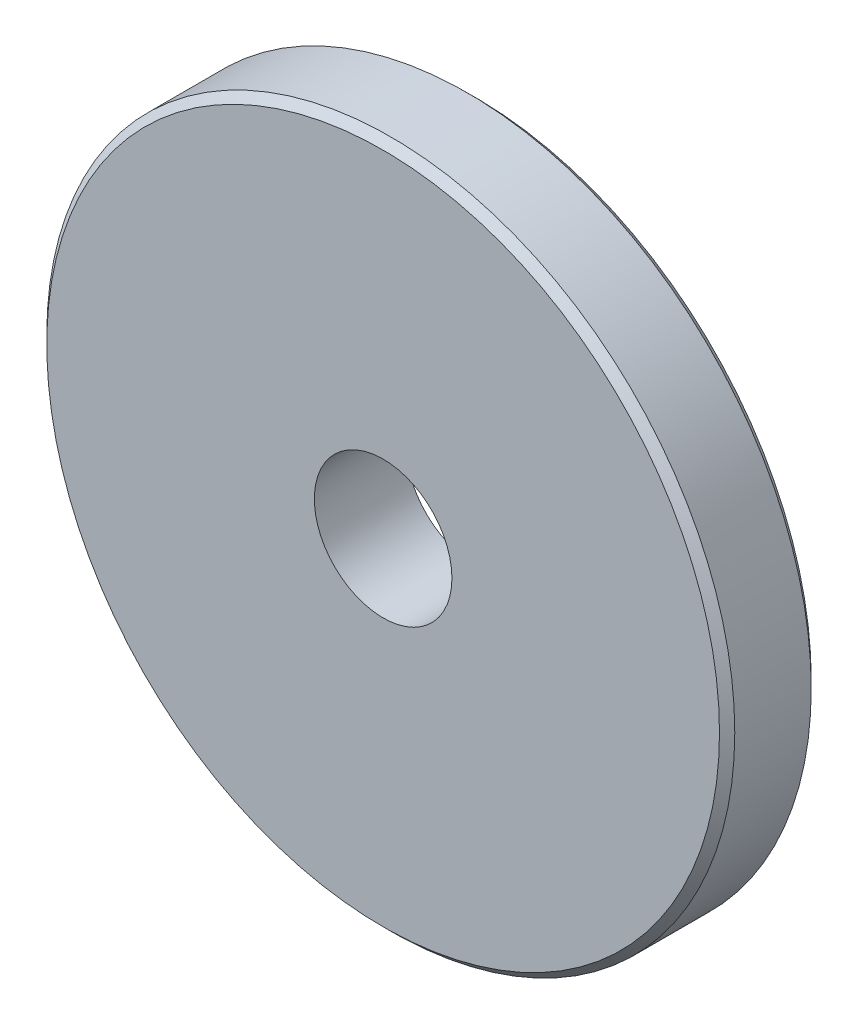
SolidWorks part; units mm, degrees
ref_plane "前视基准面" through (0, 0, 0) normal (0, 0, 1) x (1, 0, 0)
ref_plane "上视基准面" through (0, 0, 0) normal (0, 1, 0) x (1, 0, 0)
ref_plane "右视基准面" through (0, 0, 0) normal (1, 0, 0) x (0, 0, -1)
other "Configuration Table"
sketch "草图1" plane through (0, 0, 0) normal (0, 0, 1) x (1, 0, 0)
  circle A0 centre (0, 0) radius 22.5
  circle A1 centre (0, 0) radius 4.5
  dimension "D1" = 9
  dimension "D2" = 45
extrude "凸台-拉伸1" add sketch "草图1" along normal blind 6
chamfer "倒角1" distance 0.5 angle 45 2 edges at (22.5, 0, 0) (22.5, 0, 6)
